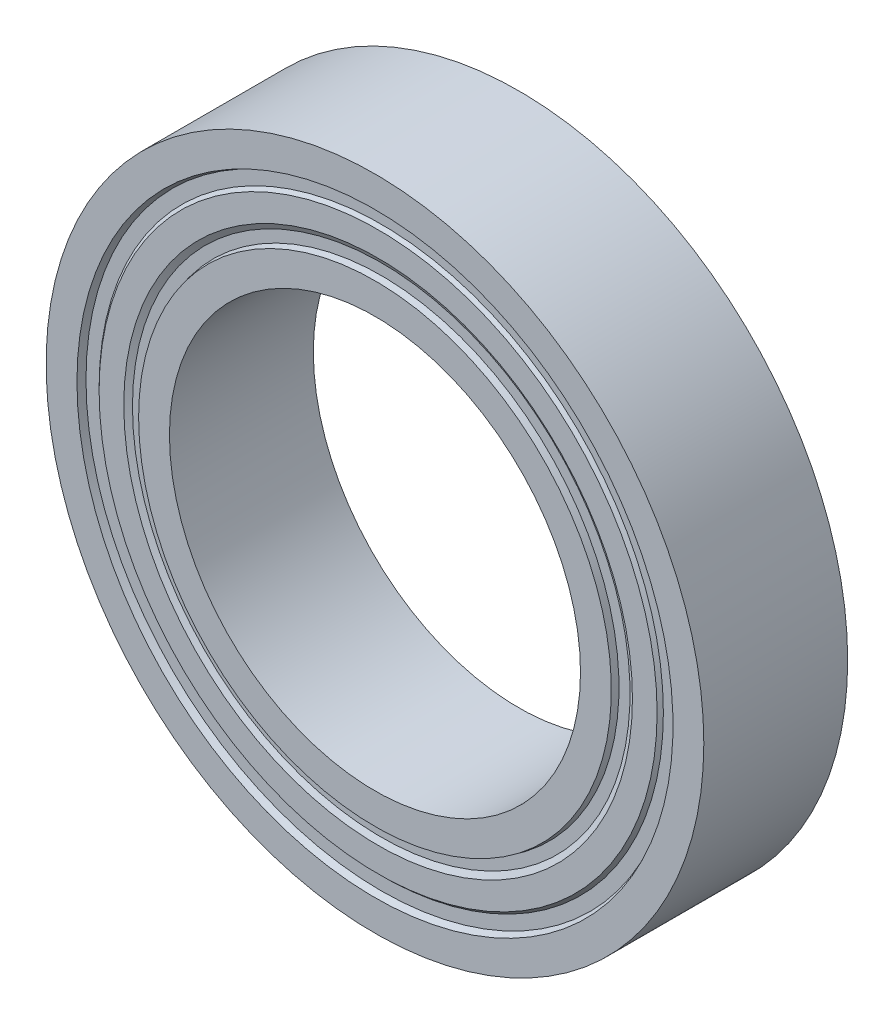
SolidWorks part; units mm, degrees
ref_plane "Front Plane" through (0, 0, 0) normal (0, 0, 1) x (1, 0, 0)
ref_plane "Top Plane" through (0, 0, 0) normal (0, 1, 0) x (1, 0, 0)
ref_plane "Right Plane" through (0, 0, 0) normal (1, 0, 0) x (0, 0, -1)
sketch "Sketch1" plane through (0, 0, 0) normal (0, 0, 1) x (1, 0, 0)
  circle A0 centre (0, 0) radius 16
  circle A1 centre (0, 0) radius 10
  dimension "D1" = 32
  dimension "D2" = 20
extrude "Boss-Extrude1" add sketch "Sketch1" along normal blind 7
sketch "Sketch3" plane through (0, 0, 0) normal (0, 1, 0) x (1, 0, 0)
  line L0 (0, 0) -> (0, -13.7899) construction
  line L1 (11.5, -7) -> (11.5673, -6.6946)
  line L2 (-16, -7) -> (16, -7) construction
  line L3 (11.5673, -6.6946) -> (12.1053, -6.6946)
  line L4 (12.1053, -6.6946) -> (12.3747, -6.8473)
  line L5 (12.3747, -6.8473) -> (13.5747, -6.8473)
  line L6 (13.5747, -6.8473) -> (13.7274, -6.6946)
  line L7 (13.7274, -6.6946) -> (14.366, -6.6946)
  line L8 (14.366, -6.6946) -> (14.5, -7)
  line L9 (11.5, -7) -> (14.5, -7)
  line L11 (16, -7) -> (16, 0) construction
  dimension "D1" = 1.5
  dimension "D2" = 1.5
  dimension "D3" = 1.2
revolve "Cut-Revolve1" cut sketch "Sketch3" angle 360 about L0
ref_plane "Plane1" through (0, 0, 3.5) normal (0, 0, 1) x (1, 0, 0)
mirror "Mirror1" about plane through (0, 0, 3.5) normal (0, 0, 1) of "Cut-Revolve1"
